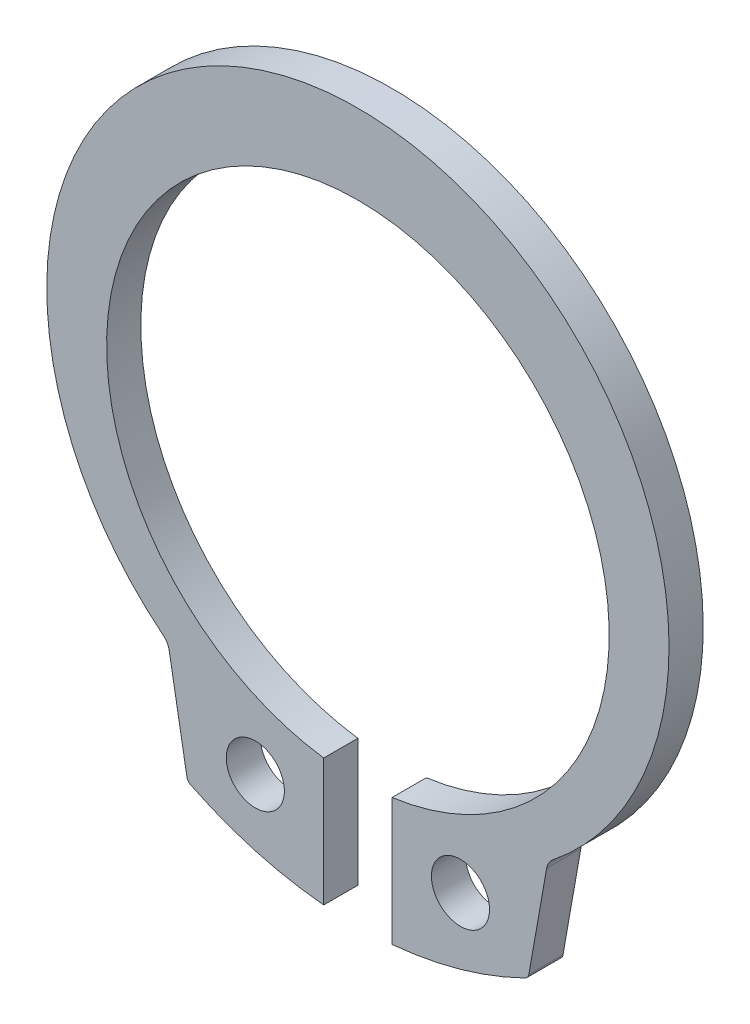
from build123d import *

# Parameters (mm, degrees)
BASE_EXTRUDE_DEPTH      = 0.5
BASE_EXTRUDE_DEPTH_BACK = 0.5
SKETCH1_R               = 0.85


with BuildPart() as part:
    # Sketch1 → Base-Extrude (new, two sides: drawn at the far end of the back side and taken through both)
    with BuildSketch(Plane.XY.offset(-BASE_EXTRUDE_DEPTH_BACK)):
        with BuildLine():
            Line((-1, -7.861655032), (-1, -11.584658105))
            ThreePointArc((-1, -11.584658105), (-2.996355114, -11.21599342), (-4.89157372, -10.488330159))
            ThreePointArc((-4.89157372, -10.488330159), (-4.963053699, -10.428973531), (-5, -10.343723502))
            Line((-5, -10.343723502), (-5.51947234, -7.397649464))
            ThreePointArc((-5.51947234, -7.397649464), (-5.581565084, -7.229851618), (-5.698757664, -7.094657221))
            ThreePointArc((-5.698757664, -7.094657221), (0, 9.1), (5.698757664, -7.094657221))
            ThreePointArc((5.698757664, -7.094657221), (5.581565084, -7.229851618), (5.51947234, -7.397649464))
            Line((5.51947234, -7.397649464), (5, -10.343723502))
            ThreePointArc((5, -10.343723502), (4.963053699, -10.428973531), (4.89157372, -10.488330159))
            ThreePointArc((4.89157372, -10.488330159), (2.996355114, -11.21599342), (1, -11.584658105))
            Line((1, -11.584658105), (1, -7.861655032))
            ThreePointArc((1, -7.861655032), (0, 6.77), (-1, -7.861655032))
        make_face()
        with Locations((-3, -9.277125962)):
            Circle(SKETCH1_R, mode=Mode.SUBTRACT)
        with Locations(Location((3, -9.277125962, 0), (0, 0, 180))):
            Circle(SKETCH1_R, mode=Mode.SUBTRACT)
    extrude(amount=BASE_EXTRUDE_DEPTH + BASE_EXTRUDE_DEPTH_BACK)


solid = part.part
